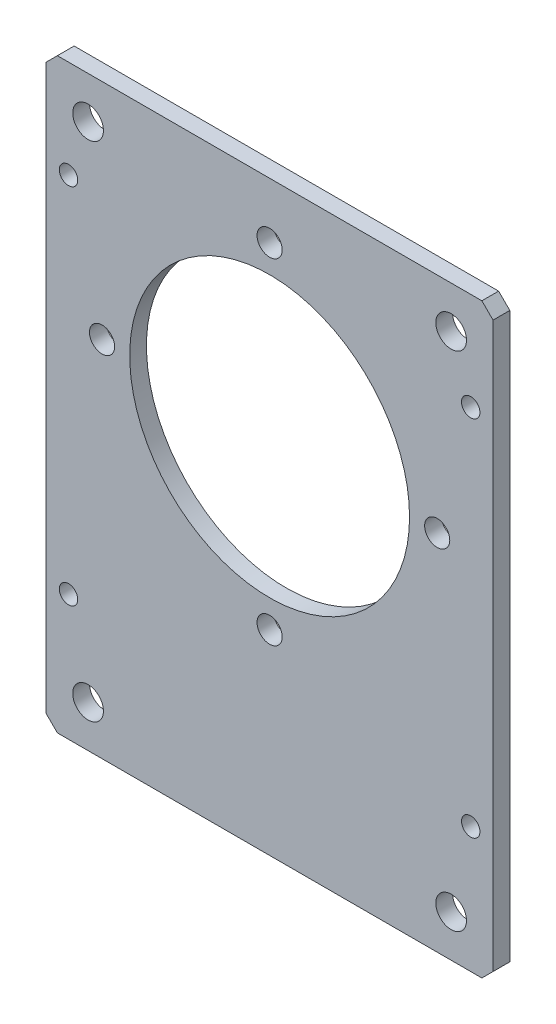
SolidWorks part; units mm, degrees
ref_plane "Front" through (0, 0, 0) normal (0, 0, 1) x (1, 0, 0)
ref_plane "Top" through (0, 0, 0) normal (0, 1, 0) x (1, 0, 0)
ref_plane "Right" through (0, 0, 0) normal (1, 0, 0) x (0, 0, -1)
sketch "Sketch1" plane through (0, 0, 0) normal (0, 0, 1) x (1, 0, 0)
  line L1 (0, 0) -> (80, 0)
  line L2 (0, 0) -> (0, 105)
  line L3 (0, 105) -> (80, 105)
  line L4 (80, 0) -> (80, 105)
  dimension "D1" = 80
  dimension "D2" = 105
extrude "Boss-Extrude1" add sketch "Sketch1" along normal blind 3
sketch "Sketch2" plane through (0, 0, 3) normal (0, 0, 1) x (1, 0, 0)
  line L0 (40, 105) -> (40, 0) construction
  line L1 (80, 105) -> (0, 105) construction
  line L2 (0, 0) -> (80, 0) construction
  line L3 (0, 52.5) -> (80, 52.5) construction
  line L4 (0, 105) -> (0, 0) construction
  line L5 (80, 0) -> (80, 105) construction
  circle A0 centre (7.5, 97.5) radius 2.75
  circle A1 centre (72.5, 97.5) radius 2.75
  circle A2 centre (72.5, 7.5) radius 2.75
  circle A3 centre (7.5, 7.5) radius 2.75
  circle A4 centre (40, 65) radius 25.05
  dimension "D1" = 5.5
  dimension "D2" = 65
  dimension "D3" = 90
  dimension "D4" = 40
  dimension "D5" = 50.1
extrude "Cut-Extrude1" cut sketch "Sketch2" against normal through all
hole_wizard "Ø4.5 (4.5) Diameter Hole1" positions "Sketch5" profile "Sketch4" hole size "Ø4.5" standard "Gb" end condition through all
sketch "Sketch5" plane through (0, 0, 3) normal (0, 0, 1) x (1, 0, 0)
  line L0 (0, 52.5) -> (80, 52.5) construction
  line L1 (0, 105) -> (0, 0) construction
  line L2 (80, 0) -> (80, 105) construction
  line L5 (40, 105) -> (40, 0) construction
  line L6 (80, 105) -> (0, 105) construction
  line L7 (0, 0) -> (80, 0) construction
  circle A0 centre (40, 65) radius 30 construction
  point P7 (40, 95)
  point P9 (10, 65)
  point P11 (70, 65)
  point P13 (40, 35)
  dimension "D1" = 60
sketch "Sketch4" plane through (40, 95, 3) normal (1, 0, 0) x (0, -1, 0)
  line L0 (0, 0) -> (0, 3)
  line L1 (0, 3) -> (2.25, 3)
  line L2 (2.25, 3) -> (2.25, 0)
  line L5 (2.25, 0) -> (0, 0)
  line L11 (0, -6.35) -> (0, 107.95) construction
  dimension "通孔孔直径" = 4.5
  dimension "通孔孔深度" = 3
chamfer "Chamfer1" distance 2 angle 45 4 edges at (80, 0, 1.5) (0, 0, 1.5) (80, 105, 1.5) (0, 105, 1.5)
hole_wizard "M4 Tapped Hole1" positions "Sketch7" profile "Sketch6" tap size "M4" standard "Gb"
sketch "Sketch7" plane through (0, 0, 3) normal (0, 0, 1) x (1, 0, 0)
  line L1 (76, 22.5) -> (4, 22.5) construction
  line L2 (76, 22.5) -> (76, 87.5) construction
  line L3 (76, 87.5) -> (4, 87.5) construction
  line L4 (4, 22.5) -> (4, 87.5) construction
  line L5 (76, 22.5) -> (4, 87.5) construction
  line L6 (76, 87.5) -> (4, 22.5) construction
  line L7 (78, 105) -> (2, 105) construction
  line L8 (40, 105) -> (40, 79.3696) construction
  point P0 (4, 87.5)
  point P2 (76, 87.5)
  point P4 (76, 22.5)
  point P6 (4, 22.5)
  point P9 (40, 65)
  dimension "D1" = 72
  dimension "D2" = 65
  dimension "D3" = 17.5
sketch "Sketch6" plane through (4, 87.5, 3) normal (1, 0, 0) x (0, -1, 0)
  line L0 (0, 0) -> (0, 11.0914)
  line L1 (0, 11.0914) -> (1.65, 10.1)
  line L2 (1.65, 10.1) -> (1.65, 0)
  line L5 (1.65, 0) -> (0, 0)
  line L10 (0, 11.0914) -> (-1.65, 10.1) construction
  line L11 (0, -6.35) -> (0, 107.95) construction
  dimension "螺纹孔钻头直径" = 3.3
  dimension "螺纹孔钻头深度" = 10.1
  dimension "导头角度" = 118
cosmetic thread "Cosmetic Thread1" parameters "D1"=3, "D2"=4
cosmetic thread "Cosmetic Thread2" parameters "D1"=3, "D2"=4
cosmetic thread "Cosmetic Thread3" parameters "D1"=3, "D2"=4
cosmetic thread "Cosmetic Thread4" parameters "D1"=3, "D2"=4
